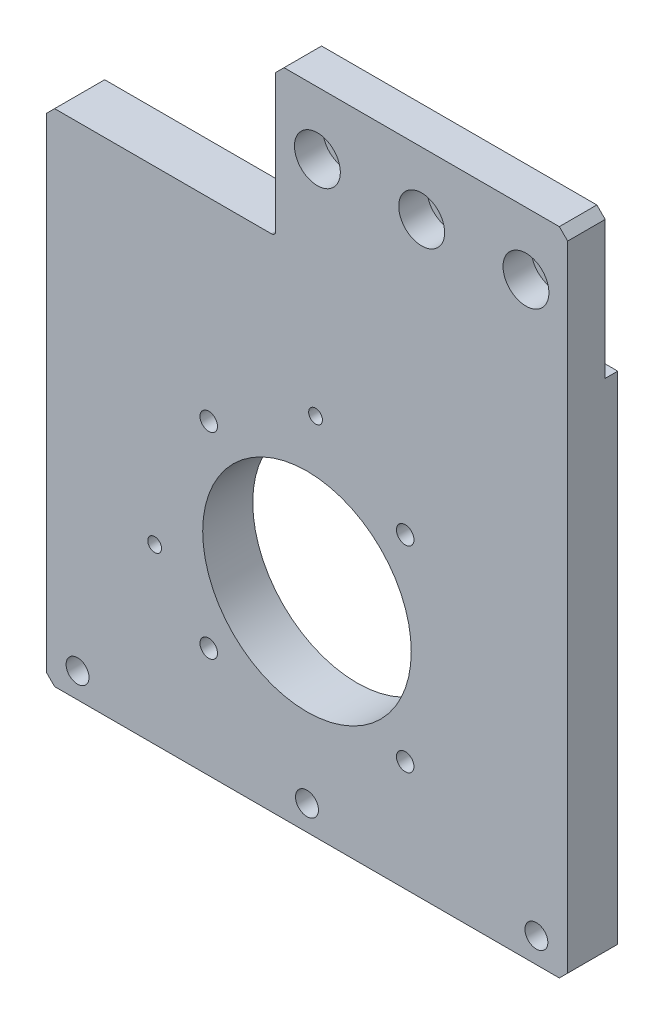
SolidWorks part; units mm, degrees
ref_plane "前视基准面" through (0, 0, 0) normal (0, 0, 1) x (1, 0, 0)
ref_plane "上视基准面" through (0, 0, 0) normal (0, 1, 0) x (1, 0, 0)
ref_plane "右视基准面" through (0, 0, 0) normal (1, 0, 0) x (0, 0, -1)
sketch "草图1" plane through (0, 0, 0) normal (0, 0, 1) x (1, 0, 0)
  line L1 (-62.5, -78) -> (62.5, -78)
  line L2 (-62.5, -78) -> (-62.5, 78)
  line L3 (-62.5, 78) -> (62.5, 78)
  line L4 (62.5, -78) -> (62.5, 78)
  line L5 (-62.5, -78) -> (62.5, 78) construction
  line L6 (-62.5, 78) -> (62.5, -78) construction
  point P0 (0, 0)
  dimension "D1" = 125
  dimension "D2" = 156
extrude "凸台-拉伸1" add sketch "草图1" along normal blind 12
sketch "草图2" plane through (0, 0, 12) normal (0, 0, 1) x (1, 0, 0)
  line L1 (-62.5, 78) -> (-7.5, 78)
  line L2 (-62.5, 78) -> (-62.5, 42)
  line L3 (-62.5, 42) -> (-7.5, 42)
  line L4 (-7.5, 78) -> (-7.5, 42)
  dimension "D1" = 55
  dimension "D2" = 36
extrude "切除-拉伸1" cut sketch "草图2" against normal through all
sketch "草图3" plane through (0, 0, 0) normal (0, 0, -1) x (-1, 0, 0)
  line L0 (7.5, 42) -> (7.5, 78) construction
  line L1 (-62.5, 78) -> (7.5, 78)
  line L2 (-62.5, 78) -> (-62.5, 43)
  line L3 (-62.5, 43) -> (7.5, 43)
  line L4 (7.5, 78) -> (7.5, 43)
  dimension "D1" = 35
extrude "切除-拉伸2" cut sketch "草图3" against normal blind 3
hole_wizard "打孔尺寸(%根据)内六角圆柱头螺钉的类型1" positions "草图4" profile "草图5" counterbore size "M5" standard "GB" end condition through all
sketch "草图4" plane through (0, 0, 0) normal (0, 0, -1) x (-1, 0, 0)
  line L0 (0, -78) -> (0, -72) construction
  line L1 (62.5, -78) -> (-62.5, -78) construction
  point P0 (-55, -72)
  point P2 (0, -72)
  point P4 (55, -72)
  point P13 (0, 0)
  point P14 (0, 0)
  dimension "D1" = 6
  dimension "D2" = 110
sketch "草图5" plane through (55, -72, 0) normal (1, 0, 0) x (0, 1, 0)
  line L0 (0, 0) -> (0, 12)
  line L1 (0, 12) -> (2.75, 12)
  line L3 (2.75, 12) -> (2.75, 5.7)
  line L4 (2.75, 5.7) -> (5, 5.7)
  line L5 (5, 5.7) -> (5, 0)
  line L7 (5, 0) -> (0, 0)
  line L11 (0, -6.35) -> (0, 107.95) construction
  dimension "通孔孔直径" = 5.5
  dimension "通孔孔深度" = 12
  dimension "柱形沉头孔直径" = 10
  dimension "柱形沉头孔深度" = 5.7
hole_wizard "打孔尺寸(%根据)内六角圆柱头螺钉的类型2" positions "草图8" profile "草图9" counterbore size "M6" standard "GB" end condition through all
sketch "草图8" plane through (0, 0, 12) normal (0, 0, -1) x (-1, 0, 0)
  line L1 (-27.5, 78) -> (-27.5, 43) construction
  line L2 (7.5, 78) -> (-62.5, 78) construction
  line L3 (-62.5, 43) -> (7.5, 43) construction
  line L5 (-62.5, 43) -> (7.5, 43) construction
  point P0 (-52.5, 63)
  point P2 (-27.5, 63)
  point P4 (-2.5, 63)
  point P19 (0, 0)
  point P22 (0, 0)
  dimension "D1" = 20
  dimension "D2" = 50
sketch "草图9" plane through (52.5, 63, 12) normal (1, 0, 0) x (0, -1, 0)
  line L0 (0, 0) -> (0, 12)
  line L1 (0, 12) -> (3.3, 12)
  line L3 (3.3, 12) -> (3.3, 6.8)
  line L4 (3.3, 6.8) -> (5.5, 6.8)
  line L5 (5.5, 6.8) -> (5.5, 0)
  line L7 (5.5, 0) -> (0, 0)
  line L11 (0, -6.35) -> (0, 107.95) construction
  dimension "通孔孔直径" = 6.6
  dimension "通孔孔深度" = 12
  dimension "柱形沉头孔直径" = 11
  dimension "柱形沉头孔深度" = 6.8
chamfer "倒角1" distance 2 angle 45 5 edges at (-62.5, 42, 6) (-7.5, 78, 7.5) (62.5, 78, 7.5) (62.5, -78, 6) (-62.5, -78, 6)
fillet "圆角1" radius 1 1 edges at (-7.5, 42, 6)
sketch "草图10" plane through (0, 0, 12) normal (0, 0, 1) x (1, 0, 0)
  line L0 (0, -78) -> (0, -28) construction
  line L1 (-60.5, -78) -> (60.5, -78) construction
  circle A0 centre (0, -28) radius 25
  point P7 (0, 0)
  dimension "D1" = 50
  dimension "D2" = 50
extrude "切除-拉伸3" cut sketch "草图10" against normal through all
hole_wizard "M5 螺纹孔1" positions "草图11" profile "草图12" tap size "M5" standard "GB" end condition through all
sketch "草图11" plane through (0, 0, 0) normal (0, 0, -1) x (-1, 0, 0)
  point P0 (-23.55, -4.45)
  point P3 (23.55, -4.45)
  point P6 (23.55, -51.55)
  point P9 (-23.55, -51.55)
sketch "草图12" plane through (23.55, -4.45, 0) normal (1, 0, 0) x (0, 1, 0)
  line L0 (0, 0) -> (0, 12)
  line L1 (0, 12) -> (2.1, 12)
  line L2 (2.1, 12) -> (2.1, 0)
  line L5 (2.1, 0) -> (0, 0)
  line L11 (0, -6.35) -> (0, 107.95) construction
  dimension "通孔螺纹孔钻头直径" = 4.2
  dimension "通孔螺纹孔钻头深度" = 12
cosmetic thread "孔螺蚊线1" parameters "D2"=5
cosmetic thread "孔螺蚊线2" parameters "D2"=5
cosmetic thread "孔螺蚊线3" parameters "D2"=5
cosmetic thread "孔螺蚊线4" parameters "D2"=5
hole_wizard "M4 螺纹孔1" positions "草图13" profile "草图14" tap size "M4" standard "GB" end condition through all
sketch "草图13" plane through (0, 0, 12) normal (0, 0, 1) x (1, 0, 0)
  line L0 (-39.5847, -33.9414) -> (-33.4571, -39.0846) construction
  line L2 (-1.0104, 12.0154) -> (5.1172, 6.8721) construction
  point P0 (2.0534, 9.4437)
  point P2 (-36.5209, -36.513)
  point P17 (2.7125, 9.4018)
sketch "草图14" plane through (2.0534, 9.4437, 12) normal (1, 0, 0) x (0, -1, 0)
  line L0 (0, 0) -> (0, 12)
  line L1 (0, 12) -> (1.65, 12)
  line L2 (1.65, 12) -> (1.65, 0)
  line L5 (1.65, 0) -> (0, 0)
  line L11 (0, -6.35) -> (0, 107.95) construction
  dimension "通孔螺纹孔钻头直径" = 3.3
  dimension "通孔螺纹孔钻头深度" = 12
cosmetic thread "孔螺蚊线5" parameters "D2"=4
cosmetic thread "孔螺蚊线6" parameters "D2"=4
